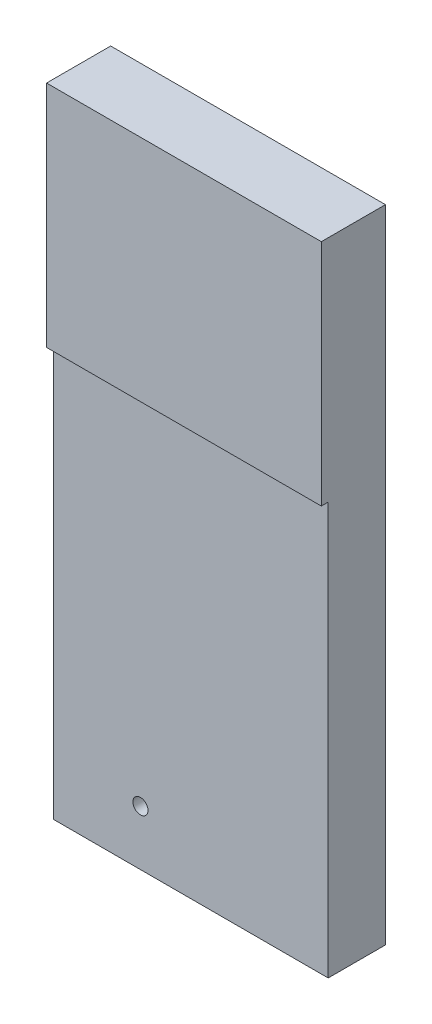
from build123d import *

# Parameters (mm, degrees)
SKETCH_1_W          = 60
SKETCH_1_H          = 140
EXTRUDE_1_DEPTH     = 14
SKETCH_2_W          = 60
SKETCH_2_H          = 90
CUT_EXTRUDE_1_DEPTH = 1.5
HOLE_WIZARD_M4_1_D  = 3.3


with BuildPart() as part:
    # 草图1 → 凸台-拉伸1 (new body)
    with BuildSketch(Plane.XY):
        Rectangle(SKETCH_1_W, SKETCH_1_H)
    extrude(amount=EXTRUDE_1_DEPTH)

    # 草图2 → 切除-拉伸1 (cut)
    with BuildSketch(Plane.XY.offset(14)):
        with Locations((0, -25)):
            Rectangle(SKETCH_2_W, SKETCH_2_H)
    extrude(amount=-CUT_EXTRUDE_1_DEPTH, mode=Mode.SUBTRACT)

    # M4 螺纹孔1 (through all)
    with Locations(Plane(origin=(0, 0, 0), x_dir=(-1, 0, 0), z_dir=(0, 0, -1))):
        with Locations((11, -58)):
            Hole(HOLE_WIZARD_M4_1_D / 2)


solid = part.part
